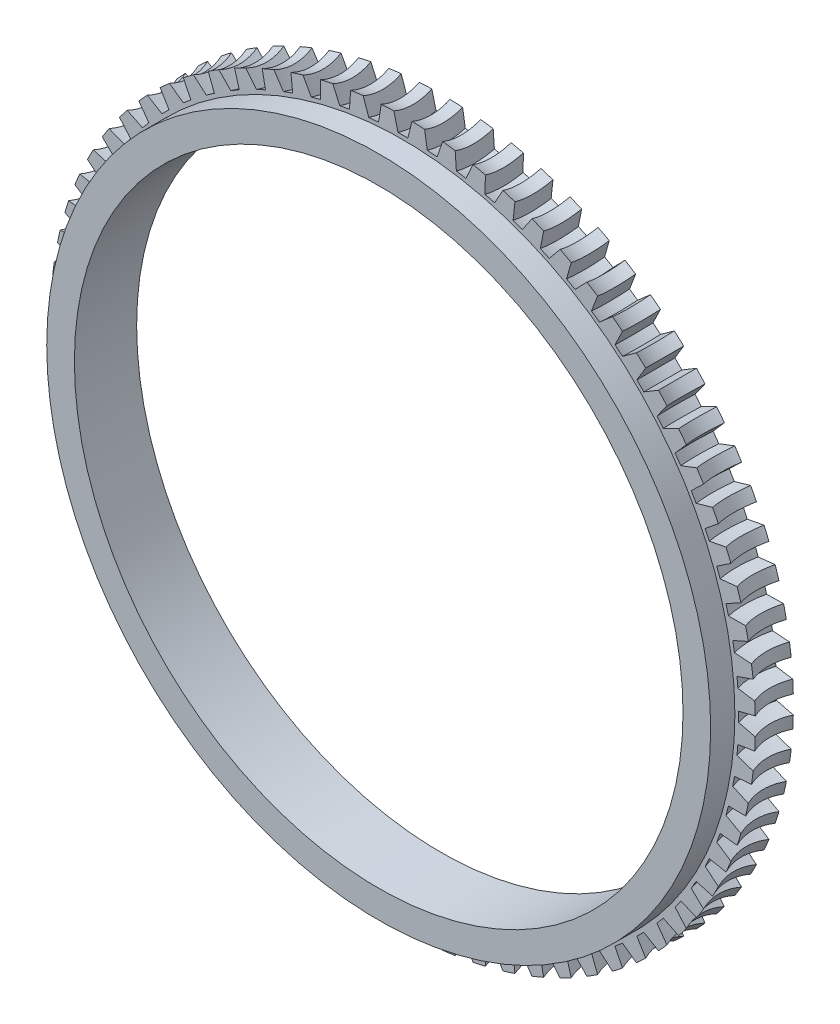
SolidWorks part; units mm, degrees
ref_plane "Front Plane" through (0, 0, 0) normal (0, 0, 1) x (1, 0, 0)
ref_plane "Top Plane" through (0, 0, 0) normal (0, 1, 0) x (1, 0, 0)
ref_plane "Right Plane" through (0, 0, 0) normal (1, 0, 0) x (0, 0, -1)
other "Configuration Table"
ref_plane "Plane1" through (0, 318.5, 0) normal (0, -1, 0) x (-1, 0, 0)
sketch "Sketch1" plane through (0, 318.5, 0) normal (0, -1, 0) x (-1, 0, 0)
  line L0 (0, 0) -> (0, 152.9236) construction
  line L1 (203, 157.0288) -> (203, -44.1767) construction
  line L2 (171, 102.5) -> (228.5, 102.5) construction
  line L4 (228.5, 102.5) -> (228.5, -53.974) construction
  line L5 (171, 77.5) -> (171, 127.5) construction
  line L6 (176, 77.5) -> (192, 77.5)
  line L7 (176, 113.5) -> (203.8423, 113.5)
  line L8 (176, 113.5) -> (176, 77.5)
  line L10 (192, 91.5) -> (203.8423, 91.5)
  line L11 (192, 91.5) -> (192, 77.5)
  arc A0 (203.8423, 113.5) -> (203.8423, 91.5) centre (228.5, 102.5) ccw
  arc A1 (193.697, 113.5) -> (193.697, 91.5) centre (228.5, 102.5) ccw construction
  point P14 (199.75, 102.5)
  dimension "D3" = 54
  dimension "D4" = 73
  dimension "D1" = 203
  dimension "D2" = 228.5
  dimension "D5" = 25
  dimension "D6" = 11
  dimension "D7" = 27
  dimension "D9" = 11
revolve "Revolve1" add sketch "Sketch1" angle 360 about L0
ref_plane "Plane2" through (0, 0, -102.5) normal (0, 0, -1) x (-1, 0, 0)
sketch "Sketch2" plane through (0, 0, -102.5) normal (0, 0, -1) x (-1, 0, 0)
  line L0 (0, 318.5) -> (0, 31.6569) construction
  line L1 (-4.3025, 199.1899) -> (-4.3025, 31.6569) construction
  line L2 (4.3025, 212.2313) -> (4.3025, 13.5995) construction
  line L3 (2.8357, 126.0209) -> (5.8999, 114.5853)
  line L4 (-2.8357, 126.0209) -> (-5.8999, 114.5853)
  circle A0 centre (0, 318.5) radius 198 construction
  arc A1 (-2.8357, 126.0209) -> (2.8357, 126.0209) centre (0, 318.5) ccw
  arc A2 (-5.8999, 114.5853) -> (5.8999, 114.5853) centre (0, 318.5) ccw
  dimension "D1" = 396
  dimension "D2" = 4.3025
  dimension "D5" = 385
  dimension "D6" = 408
  dimension "D3" = 4.3025
  dimension "D4" = 15
sketch "Sketch3" plane through (0, 0, 0) normal (1, 0, 0) x (0, 0, -1)
  line L0 (102.5, 318.5) -> (312.2051, 318.5) construction
  line L1 (102.5, 120.5) -> (102.5, 516.5) construction
  line L2 (102.5, 90) -> (189.288, 90) construction
  line L3 (102.5, 199.1899) -> (102.5, 31.6569) construction
  line L4 (82.6689, 93.7942) -> (82.6689, 120) construction
  line L5 (121.9544, 90) -> (121.9544, 126.7247) construction
  arc A0 (121.9544, 112.837) -> (82.6689, 112.5106) centre (102.5, 90) ccw
  dimension "D2" = 60
  dimension "D1" = 228.5
sweep "Cut-Sweep1" cut profiles "Sketch2" path "Sketch3"
pattern_circular "CirPattern1" count 72 every 5 about axis through (0, 318.5, 0) along (0, 0, 1) of "Cut-Sweep1"
